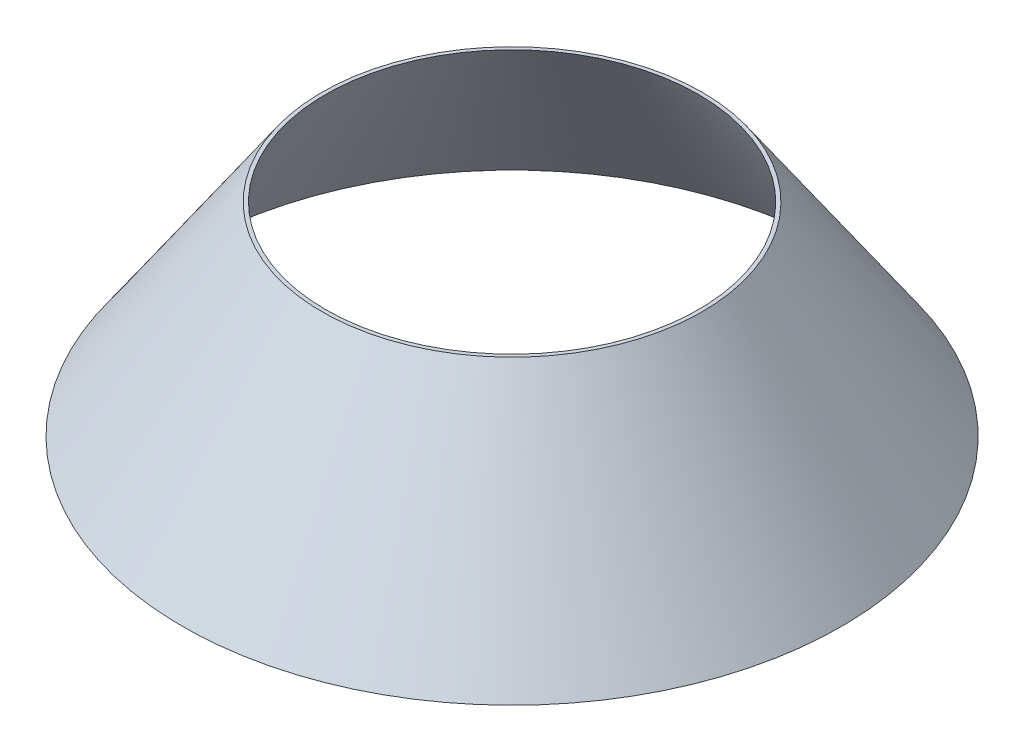
SolidWorks part; units mm, degrees
material "Q235"
ref_plane "Front Plane" through (0, 0, 0) normal (0, 0, 1) x (1, 0, 0)
ref_plane "Top Plane" through (0, 0, 0) normal (0, 1, 0) x (1, 0, 0)
ref_plane "Right Plane" through (0, 0, 0) normal (1, 0, 0) x (0, 0, -1)
sketch "Sketch3" plane through (0, 0, 0) normal (0, 0, 1) x (1, 0, 0)
  line L0 (0, 0) -> (0, 80) construction
  line L1 (0, 80) -> (75, 80)
  line L2 (75, 80) -> (130, 0)
  line L3 (130, 0) -> (0, 0)
  line L4 (0, 0) -> (0, 80)
  dimension "D1" = 150
  dimension "D2" = 260
  dimension "D3" = 80
revolve "Revolve1" add sketch "Sketch3" angle 360 about L0
shell "Shell1" thickness 1.2
